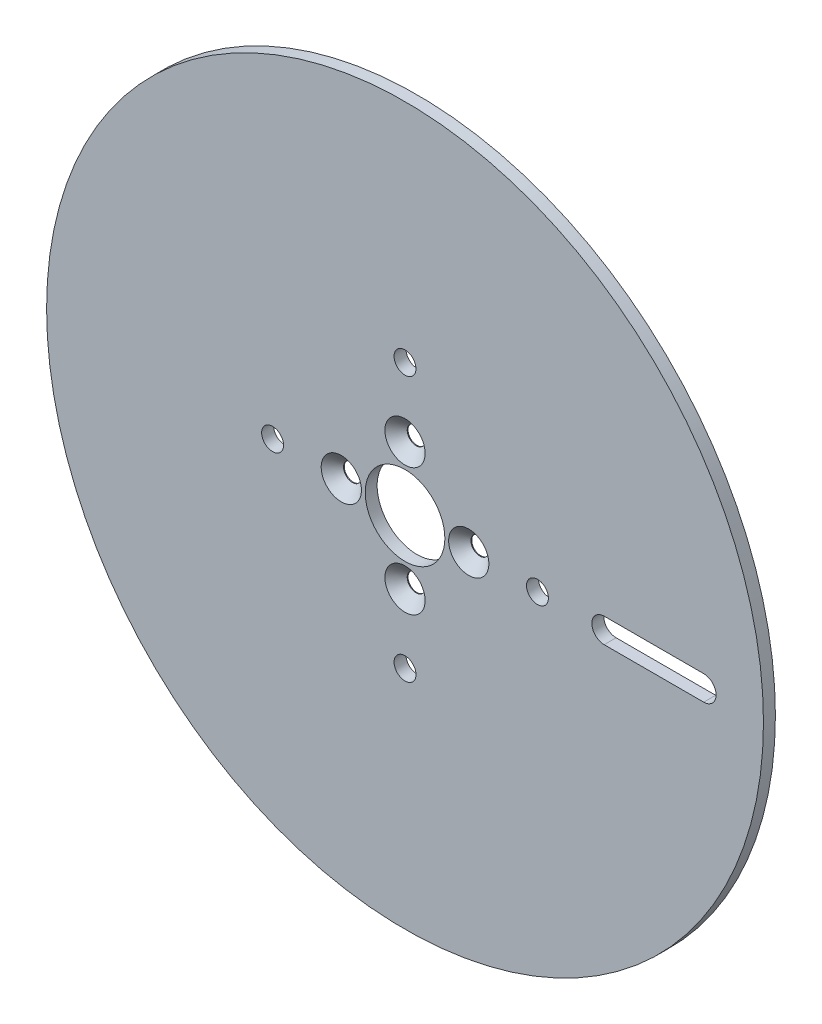
from build123d import *

# Parameters (mm, degrees)
SKETCH1_R           = 90
SKETCH1_R_2         = 10
BOSS_EXTRUDE1_DEPTH = 3
SKETCH2_R           = 2.25
SKETCH2_R_2         = 2.75
CUT_EXTRUDE1_DEPTH  = 3
CHAMFER1_SIZE       = 2.8


with BuildPart() as part:
    # Sketch1 → Boss-Extrude1 (new body)
    with BuildSketch(Plane.XY):
        Circle(SKETCH1_R)
        Circle(SKETCH1_R_2, mode=Mode.SUBTRACT)
    extrude(amount=BOSS_EXTRUDE1_DEPTH)

    # Sketch2 → Cut-Extrude1 (cut)
    with BuildSketch(Plane.XY.offset(3)):
        with Locations((0, 16)):
            Circle(SKETCH2_R)
        with Locations((-16, 0)):
            Circle(SKETCH2_R)
        with Locations((0, -16)):
            Circle(SKETCH2_R)
        with Locations((16, 0)):
            Circle(SKETCH2_R)
        with Locations((0, 33.25)):
            Circle(SKETCH2_R_2)
        with Locations((-33.25, 0)):
            Circle(SKETCH2_R_2)
        with Locations((0, -33.25)):
            Circle(SKETCH2_R_2)
        with Locations((33.25, 0)):
            Circle(SKETCH2_R_2)
        with BuildLine():
            Line((50, 3.1), (75, 3.1))
            ThreePointArc((75, 3.1), (78.1, 0), (75, -3.1))
            Line((75, -3.1), (50, -3.1))
            ThreePointArc((50, -3.1), (46.9, 0), (50, 3.1))
        make_face()
    extrude(amount=-CUT_EXTRUDE1_DEPTH, mode=Mode.SUBTRACT)

    # Chamfer1
    chamfer1_edges = [part.edges().sort_by_distance(p)[0] for p in [
        (-2.25, 16, 3),
        (-18.25, 0, 3),
        (-2.25, -16, 3),
        (13.75, 0, 3),
    ]]
    chamfer(chamfer1_edges, length=CHAMFER1_SIZE)


solid = part.part
